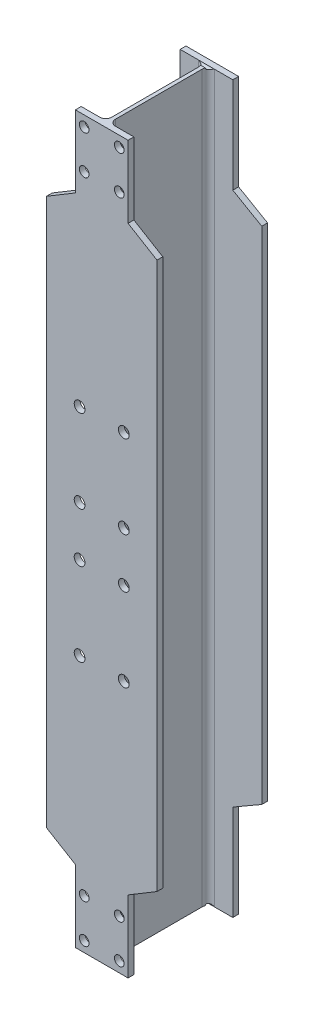
from build123d import *

# Parameters (mm, degrees)
EXTRUDE1_DEPTH     = 1312.5
CUT_EXTRUDE2_DEPTH = 30
CUT_EXTRUDE3_DEPTH = 30
SKETCH2_R          = 19.5
SKETCH2_R_2        = 17.5
CUT_EXTRUDE1_DEPTH = 50.8
SKETCH6_R          = 6.35
CUT_EXTRUDE4_DEPTH = 30


with BuildPart() as part:
    # Sketch1 → Extrude1 (new, symmetric)
    with BuildSketch(Plane(origin=(0, 0, 0), x_dir=(1, 0, 0), z_dir=(0, 1, 0))):
        with BuildLine():
            Line((-6.5, -157), (-6.5, 157))
            ThreePointArc((-6.5, 157), (-12.943650814, 172.556349186), (-28.5, 179))
            Line((-28.5, 179), (-200, 179))
            Line((-200, 179), (-200, 200))
            Line((-200, 200), (200, 200))
            Line((200, 200), (200, 179))
            Line((200, 179), (28.5, 179))
            ThreePointArc((28.5, 179), (12.943650814, 172.556349186), (6.5, 157))
            Line((6.5, 157), (6.5, -157))
            ThreePointArc((6.5, -157), (12.943650814, -172.556349186), (28.5, -179))
            Line((28.5, -179), (200, -179))
            Line((200, -179), (200, -200))
            Line((200, -200), (-200, -200))
            Line((-200, -200), (-200, -179))
            Line((-200, -179), (-28.5, -179))
            ThreePointArc((-28.5, -179), (-12.943650814, -172.556349186), (-6.5, -157))
        make_face()
    extrude(amount=EXTRUDE1_DEPTH, both=True)

    # Sketch3 → Cut-Extrude2 (cut)
    with BuildSketch(Plane.XY.offset(200)):
        Polygon((-95.25, 1312.5), (-95.25, 1052.15), (-200, 989.209850157), (-200, 1312.5), align=None)
        Polygon((95.25, 1052.15), (200, 989.209850157), (200, 1312.5), (95.25, 1312.5), align=None)
        Polygon((200, -989.209850157), (200, -1312.5), (95.25, -1312.5), (95.25, -1052.15), align=None)
        Polygon((-200, -1312.5), (-95.25, -1312.5), (-95.25, -1052.15), (-200, -989.209850157), align=None)
    extrude(amount=-CUT_EXTRUDE2_DEPTH, mode=Mode.SUBTRACT)

    # Sketch5 → Cut-Extrude3 (cut)
    with BuildSketch(Plane(origin=(0, 0, -200), x_dir=(-1, 0, 0), z_dir=(0, 0, -1))):
        Polygon((-200, 1312.5), (-95.25, 1312.5), (-95.25, 966.425), (-200, 905.947559302), align=None)
        Polygon((200, 905.947559302), (200, 1312.5), (95.25, 1312.5), (95.25, 966.425), align=None)
        Polygon((200, -1312.5), (95.25, -1312.5), (95.25, -966.425), (200, -905.947559302), align=None)
        Polygon((-200, -905.947559302), (-200, -1312.5), (-95.25, -1312.5), (-95.25, -966.425), align=None)
    extrude(amount=-CUT_EXTRUDE3_DEPTH, mode=Mode.SUBTRACT)

    # Sketch2 → Cut-Extrude1 (cut)
    with BuildSketch(Plane.XY.offset(200)):
        with Locations((-80, 390)):
            Circle(SKETCH2_R)
        with Locations((80, 390)):
            Circle(SKETCH2_R)
        with Locations((80, -390)):
            Circle(SKETCH2_R)
        with Locations((-80, -390)):
            Circle(SKETCH2_R)
        with Locations((63.5, 1274.5)):
            Circle(SKETCH2_R_2)
        with Locations((63.5, 1134.5)):
            Circle(SKETCH2_R_2)
        with Locations((-63.5, 1274.5)):
            Circle(SKETCH2_R_2)
        with Locations((-63.5, 1134.5)):
            Circle(SKETCH2_R_2)
        with Locations((63.5, -1134.5)):
            Circle(SKETCH2_R_2)
        with Locations((-63.5, -1134.5)):
            Circle(SKETCH2_R_2)
        with Locations((63.5, -1274.5)):
            Circle(SKETCH2_R_2)
        with Locations((-63.5, -1274.5)):
            Circle(SKETCH2_R_2)
        with Locations((-80, 90)):
            Circle(SKETCH2_R)
        with Locations((80, 90)):
            Circle(SKETCH2_R)
        with Locations((-80, -90)):
            Circle(SKETCH2_R)
        with Locations((80, -90)):
            Circle(SKETCH2_R)
    extrude(amount=-CUT_EXTRUDE1_DEPTH, mode=Mode.SUBTRACT)

    # Sketch6 → Cut-Extrude4 (cut, symmetric)
    with BuildSketch(Plane(origin=(0, 0, 0), x_dir=(0, 0, -1), z_dir=(1, 0, 0))):
        with Locations((172.65, 1312.5)):
            Circle(SKETCH6_R)
        with Locations((172.65, -1312.5)):
            Circle(SKETCH6_R)
    extrude(amount=CUT_EXTRUDE4_DEPTH, both=True, mode=Mode.SUBTRACT)


solid = part.part
